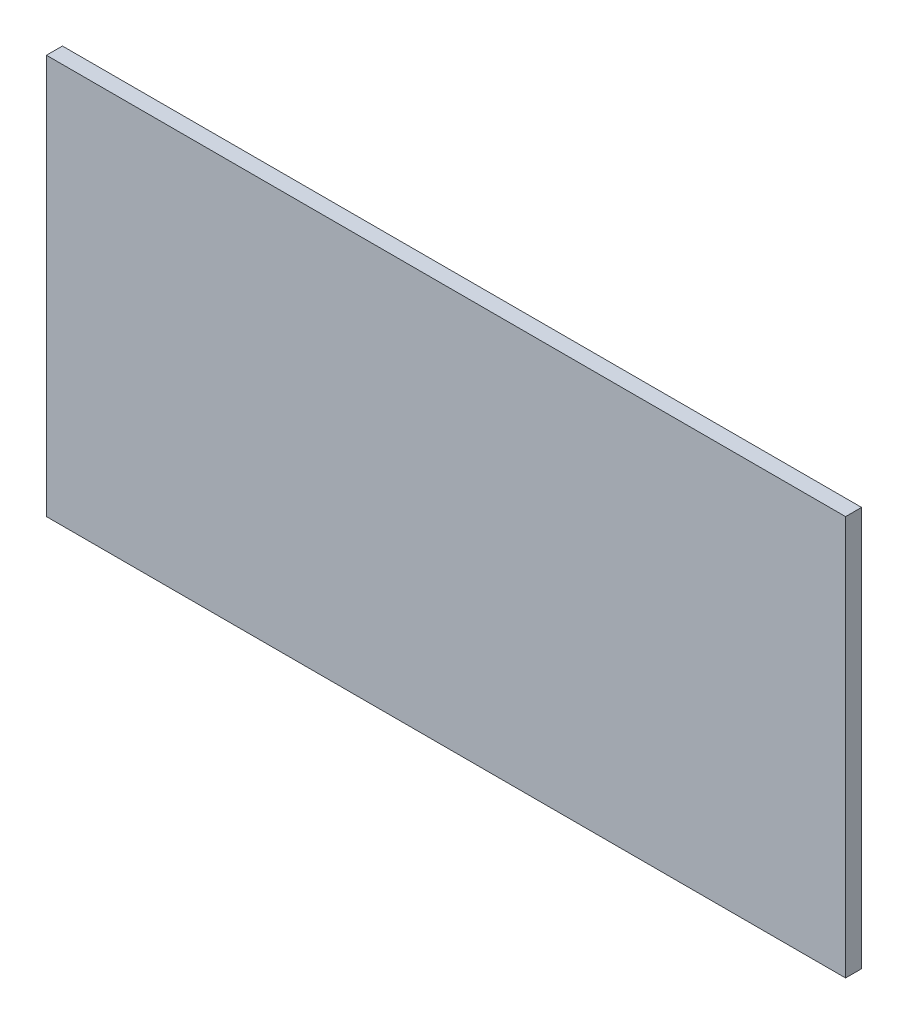
from build123d import *

# Parameters (mm, degrees)
SKETCH1_W           = 100
SKETCH1_H           = 50
BOSS_EXTRUDE1_DEPTH = 2


with BuildPart() as part:
    # Sketch1 → Boss-Extrude1 (new body)
    with BuildSketch(Plane.XY):
        Rectangle(SKETCH1_W, SKETCH1_H)
    extrude(amount=BOSS_EXTRUDE1_DEPTH)


solid = part.part
